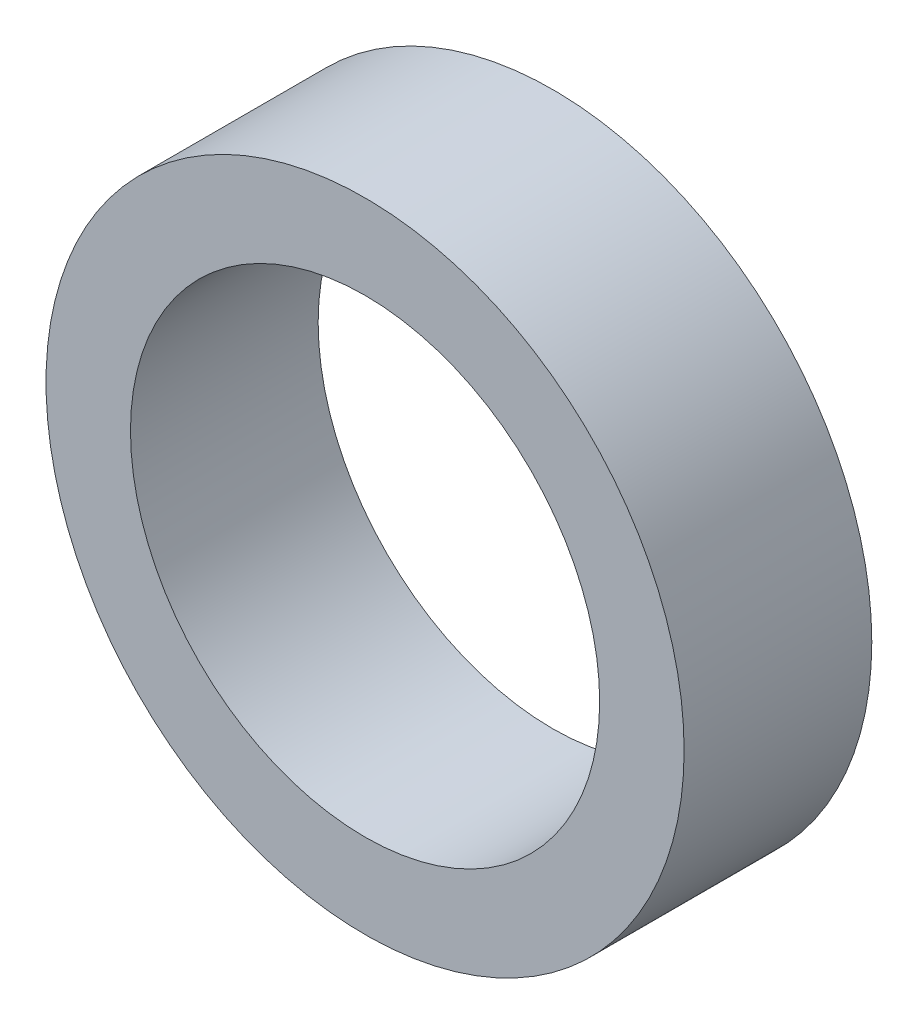
SolidWorks part; units mm, degrees
ref_plane "前视基准面" through (0, 0, 0) normal (0, 0, 1) x (1, 0, 0)
ref_plane "上视基准面" through (0, 0, 0) normal (0, 1, 0) x (1, 0, 0)
ref_plane "右视基准面" through (0, 0, 0) normal (1, 0, 0) x (0, 0, -1)
sketch "草图1" plane through (0, 0, 0) normal (0, 0, 1) x (1, 0, 0)
  circle A0 centre (0, 0) radius 6.25
  circle A1 centre (0, 0) radius 8.5
  dimension "D1" = 12.5
  dimension "D2" = 17
extrude "凸台-拉伸1" add sketch "草图1" along normal blind 5
